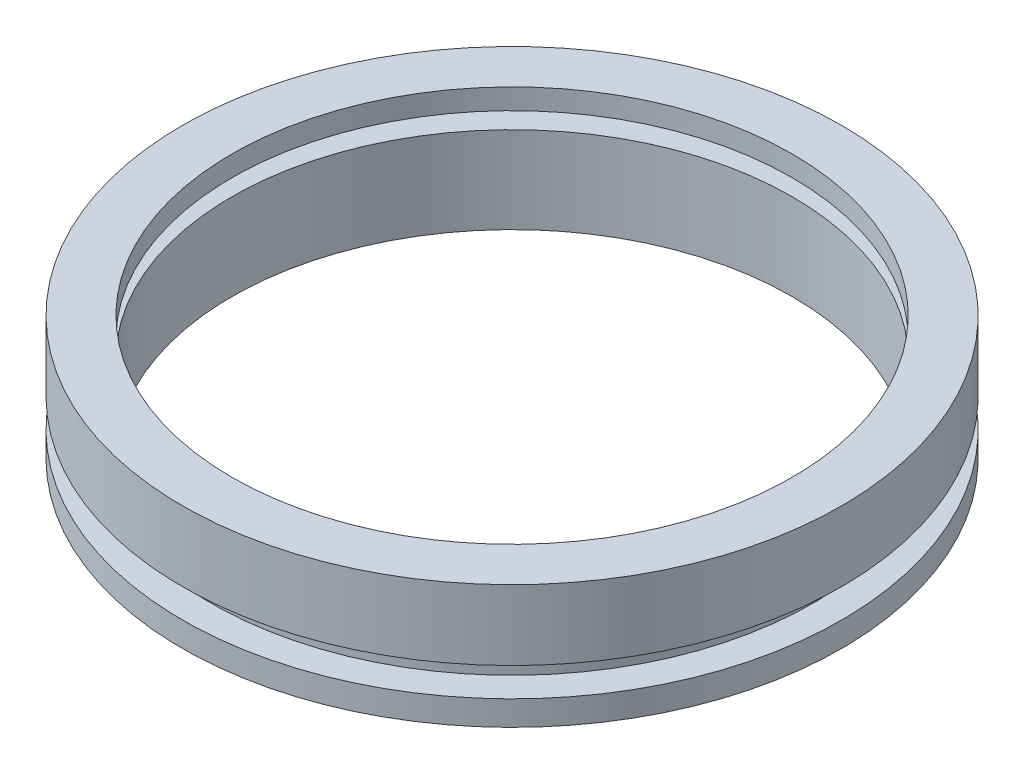
SolidWorks part; units mm, degrees
ref_plane "前视基准面" through (0, 0, 0) normal (0, 0, 1) x (1, 0, 0)
ref_plane "上视基准面" through (0, 0, 0) normal (0, 1, 0) x (1, 0, 0)
ref_plane "右视基准面" through (0, 0, 0) normal (1, 0, 0) x (0, 0, -1)
sketch "草图1" plane through (0, 0, 0) normal (0, 0, 1) x (1, 0, 0)
  line L0 (34, 0) -> (34, 27.6869) construction
  line L1 (0, 0) -> (-6, 0)
  line L2 (0, 0) -> (0, 15) construction
  line L3 (0, 15) -> (-6, 15)
  line L4 (-6, 0) -> (-6, 15) construction
  line L5 (0, 12.5) -> (-3.5, 12.5)
  line L6 (-3.5, 12.5) -> (-3.5, 10.5)
  line L7 (-3.5, 10.5) -> (0, 10.5)
  line L8 (-6, 6.5) -> (-2.5, 6.5)
  line L9 (-2.5, 6.5) -> (-2.5, 3)
  line L10 (-2.5, 3) -> (-6, 3)
  line L11 (-6, 3) -> (-6, 0)
  line L12 (-6, 6.5) -> (-6, 15)
  line L13 (0, 10.5) -> (0, 0)
  line L14 (0, 12.5) -> (0, 15)
  dimension "D1" = 34
  dimension "D2" = 15
  dimension "D3" = 6
  dimension "D4" = 3
  dimension "D5" = 3.5
  dimension "D6" = 2
  dimension "D7" = 3.5
  dimension "D8" = 2.5
revolve "旋转1" add sketch "草图1" angle 360 about L0
equation "\"图号代码1\"= \"图号代码\""
equation "\"名称代码2\"= \"名称代码\""
